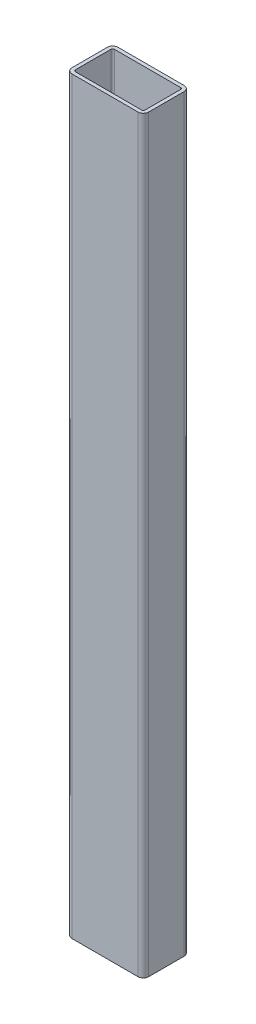
from build123d import *

# Parameters (mm, degrees)
BOSS_EXTRUDE1_DEPTH = 488


with BuildPart() as part:
    # Sketch1 → Boss-Extrude1 (new body)
    with BuildSketch(Plane(origin=(0, 0, 0), x_dir=(1, 0, 0), z_dir=(0, 1, 0))):
        with BuildLine():
            Line((-21.55, -15), (21.55, -15))
            ThreePointArc((21.55, -15), (23.989518395, -13.989518395), (25, -11.55))
            Line((25, -11.55), (25, 11.55))
            ThreePointArc((25, 11.55), (23.989518395, 13.989518395), (21.55, 15))
            Line((21.55, 15), (-21.55, 15))
            ThreePointArc((-21.55, 15), (-23.989518395, 13.989518395), (-25, 11.55))
            Line((-25, 11.55), (-25, -11.55))
            ThreePointArc((-25, -11.55), (-23.989518395, -13.989518395), (-21.55, -15))
        make_face()
        with BuildLine():
            Line((-21.55, -12.7), (21.55, -12.7))
            ThreePointArc((21.55, -12.7), (22.363172798, -12.363172798), (22.7, -11.55))
            Line((22.7, -11.55), (22.7, 11.55))
            ThreePointArc((22.7, 11.55), (22.363172798, 12.363172798), (21.55, 12.7))
            Line((21.55, 12.7), (-21.55, 12.7))
            ThreePointArc((-21.55, 12.7), (-22.363172798, 12.363172798), (-22.7, 11.55))
            Line((-22.7, 11.55), (-22.7, -11.55))
            ThreePointArc((-22.7, -11.55), (-22.363172798, -12.363172798), (-21.55, -12.7))
        make_face(mode=Mode.SUBTRACT)
    extrude(amount=BOSS_EXTRUDE1_DEPTH)


solid = part.part
